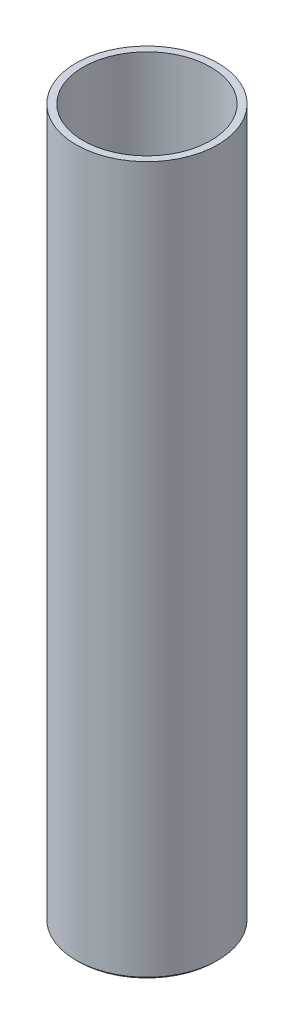
SolidWorks part; units mm, degrees
material "6061 合金"
ref_plane "Front Plane" through (0, 0, 0) normal (0, 0, 1) x (1, 0, 0)
ref_plane "Top Plane" through (0, 0, 0) normal (0, 1, 0) x (1, 0, 0)
ref_plane "Right Plane" through (0, 0, 0) normal (1, 0, 0) x (0, 0, -1)
sketch "Sketch1" plane through (0, 0, 0) normal (0, 1, 0) x (1, 0, 0)
  circle A0 centre (0, 0) radius 15
  dimension "D1" = 30
extrude "Boss-Extrude1" add sketch "Sketch1" along normal blind 150
sketch "Sketch3" plane through (0, 0, 0) normal (0, 0, 1) x (1, 0, 0)
  line L0 (0, 0) -> (0, 205.794) construction
  line L1 (15, 150) -> (-15, 150) construction
  line L2 (0, 150) -> (13.5, 150)
  line L3 (0, 150) -> (0, 2.5)
  line L4 (0, 2.5) -> (13.5, 2.5)
  line L5 (13.5, 150) -> (13.5, 2.5)
  line L6 (15, 0) -> (15, 150) construction
  line L7 (-15, 0) -> (15, 0) construction
  line L8 (0, 0) -> (13.5, 0)
  line L9 (0, 0) -> (0, 0.5)
  line L10 (0, 0.5) -> (13.5, 0.5)
  line L11 (13.5, 0) -> (13.5, 0.5)
  dimension "D1" = 1.5
  dimension "D2" = 1.5
  dimension "D3" = 0.5
  dimension "D4" = 2
revolve "Cut-Revolve1" cut sketch "Sketch3" angle 360 about L0
chamfer "Chamfer1" distance 0.5 angle 45 1 edges at (0, 0, 15)
